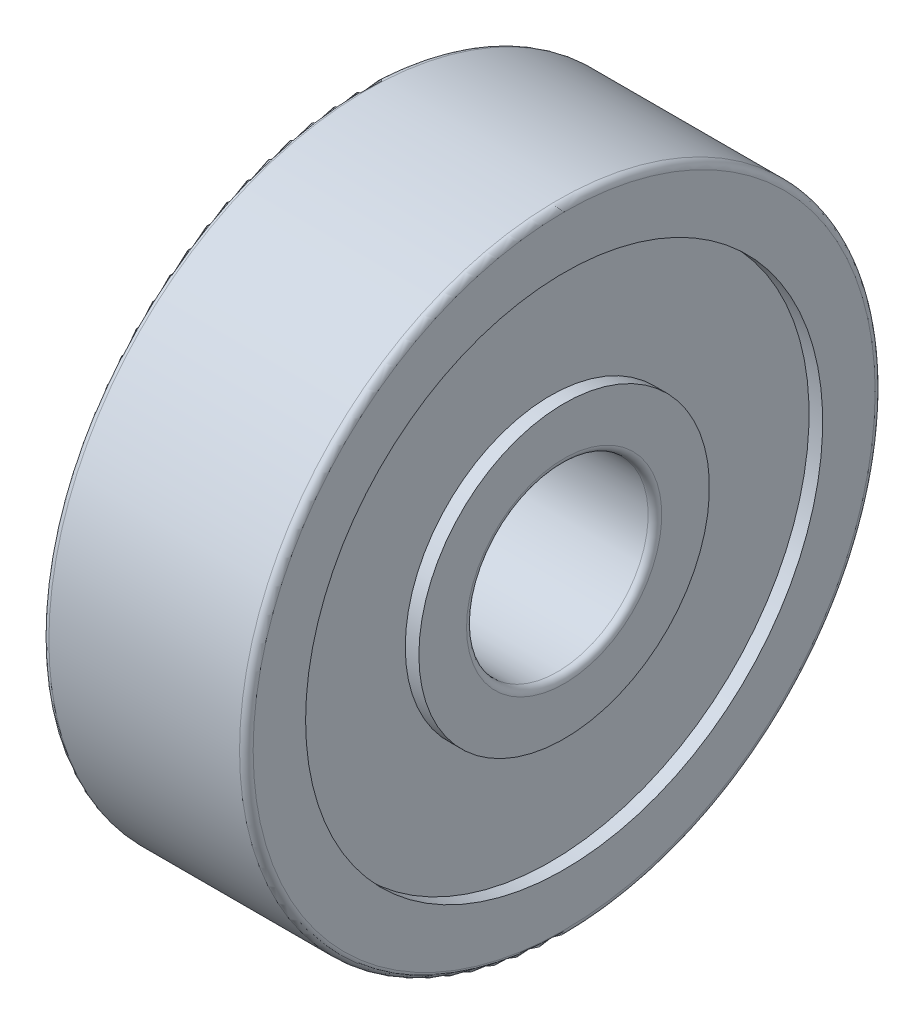
from build123d import *


with BuildPart() as part:
    # Sketch1 → Revolve1 (revolve)
    with BuildSketch(Plane.XY, mode=Mode.PRIVATE) as revolve1_sk:
        with BuildLine():
            Line((0, 11.39), (0.6, 11.39))
            Line((0.6, 11.39), (0.6, 6.4))
            Line((0.6, 6.4), (0, 6.4))
            Line((0, 6.4), (0, 4.3))
            ThreePointArc((0, 4.3), (0.087867966, 4.087867966), (0.3, 4))
            Line((0.3, 4), (8.7, 4))
            ThreePointArc((8.7, 4), (8.912132034, 4.087867966), (9, 4.3))
            Line((9, 4.3), (9, 6.4))
            Line((9, 6.4), (8.4, 6.4))
            Line((8.4, 6.4), (8.4, 11.39))
            Line((8.4, 11.39), (9, 11.39))
            Line((9, 11.39), (9, 13.7))
            ThreePointArc((9, 13.7), (8.912132034, 13.912132034), (8.7, 14))
            Line((8.7, 14), (0.3, 14))
            ThreePointArc((0.3, 14), (0.087867966, 13.912132034), (0, 13.7))
            Line((0, 13.7), (0, 11.39))
        make_face()
    revolve(revolve1_sk.sketch.rotate(Axis((-0.115, 0, 0), (1, 0, 0)), 90), axis=Axis((-0.115, 0, 0), (1, 0, 0)))


solid = part.part
